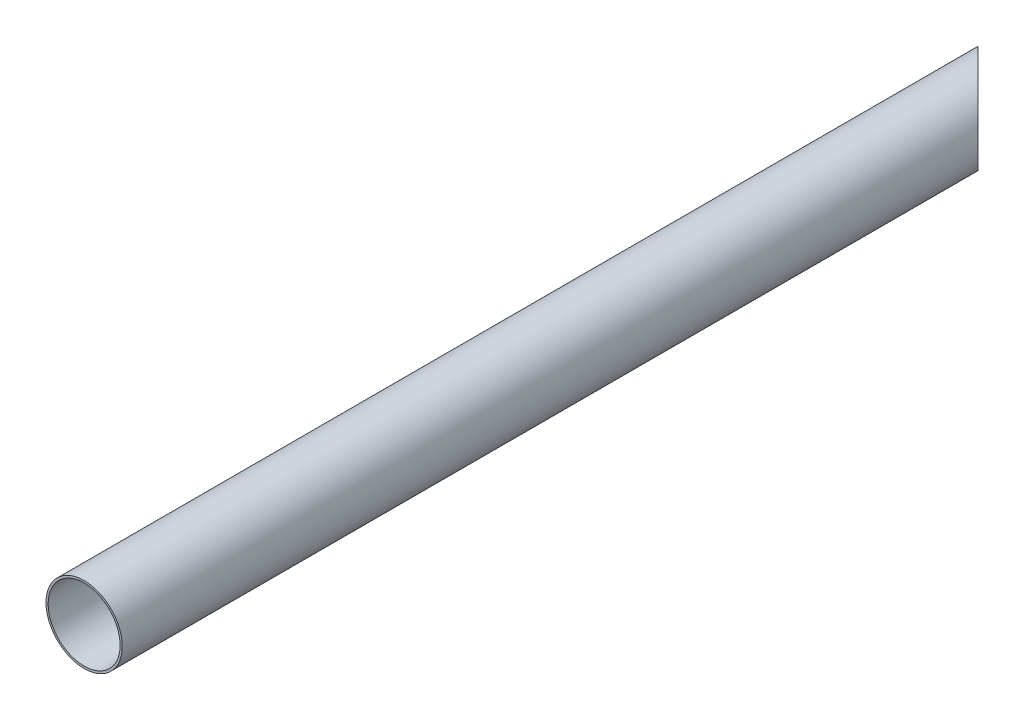
from build123d import *

# Parameters (mm, degrees)
SKETCH1_R           = 9
SKETCH1_R_2         = 8.5
BOSS_EXTRUDE1_DEPTH = 220
CUT_EXTRUDE1_DEPTH  = 110


with BuildPart() as part:
    # Sketch1 → Boss-Extrude1 (new body)
    with BuildSketch(Plane.XY):
        Circle(SKETCH1_R)
        Circle(SKETCH1_R_2, mode=Mode.SUBTRACT)
    extrude(amount=BOSS_EXTRUDE1_DEPTH)

    # Sketch2 → Cut-Extrude1 (cut, symmetric)
    with BuildSketch(Plane(origin=(0, 0, 0), x_dir=(1, 0, 0), z_dir=(0, 1, 0))):
        Polygon((-9, 0), (9, 0), (9, -18), align=None)
    extrude(amount=CUT_EXTRUDE1_DEPTH, both=True, mode=Mode.SUBTRACT)


solid = part.part
